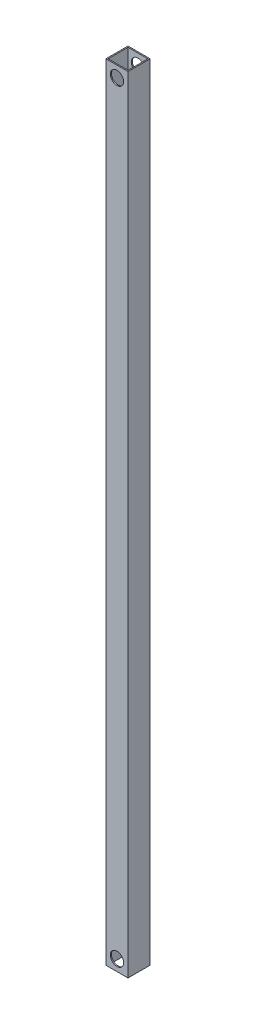
SolidWorks part; units mm, degrees
ref_plane "Front Plane" through (0, 0, 0) normal (0, 0, 1) x (1, 0, 0)
ref_plane "Top Plane" through (0, 0, 0) normal (0, 1, 0) x (1, 0, 0)
ref_plane "Right Plane" through (0, 0, 0) normal (1, 0, 0) x (0, 0, -1)
sketch "Sketch1" plane through (0, 0, 0) normal (0, 1, 0) x (1, 0, 0)
  line L0 (4.5, 4.5) -> (4.5, -4.5)
  line L1 (-5, 5) -> (5, 5)
  line L2 (-5, 5) -> (-5, -5)
  line L3 (-5, -5) -> (5, -5)
  line L4 (5, 5) -> (5, -5)
  line L5 (-5, 5) -> (5, -5) construction
  line L6 (-5, -5) -> (5, 5) construction
  line L7 (-4.5, -4.5) -> (4.5, -4.5)
  line L8 (-4.5, 4.5) -> (-4.5, -4.5)
  line L9 (-4.5, 4.5) -> (4.5, 4.5)
  point P0 (0, 0)
  dimension "D1" = 10
  dimension "D2" = 0.5
extrude "Boss-Extrude1" add sketch "Sketch1" along normal blind 355
sketch "Sketch2" plane through (0, 0, -5) normal (0, 0, -1) x (-1, 0, 0)
  line L0 (5, 355) -> (5, 0) construction
  circle A0 centre (0, 5) radius 3
  dimension "D1" = 6
  dimension "D2" = 5
  dimension "D3" = 5
extrude "Cut-Extrude1" cut sketch "Sketch2" against normal blind 19
sketch "Sketch3" plane through (0, 0, -5) normal (0, 0, -1) x (-1, 0, 0)
  line L0 (-5, 355) -> (5, 355) construction
  line L1 (5, 355) -> (5, 0) construction
  circle A0 centre (0, 350) radius 3
  dimension "D1" = 6
  dimension "D2" = 5
  dimension "D3" = 5
extrude "Cut-Extrude2" cut sketch "Sketch3" against normal blind 16
